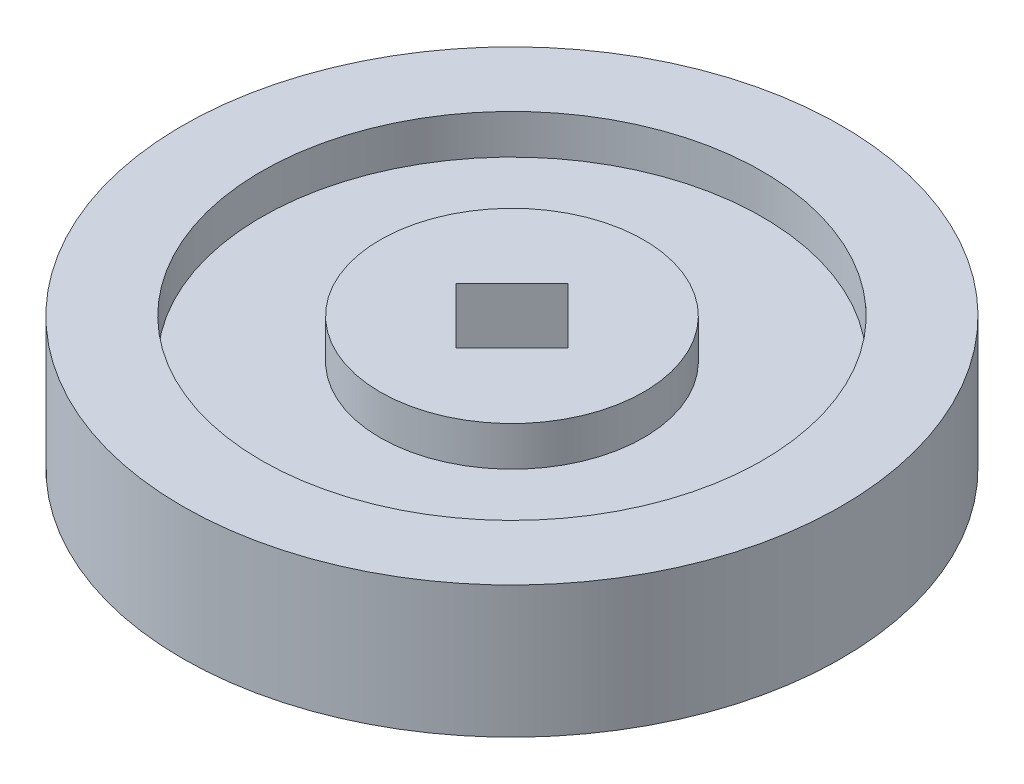
from build123d import *

# Parameters (mm, degrees)
SKETCH1_R           = 25
SKETCH1_R_2         = 19
BOSS_EXTRUDE1_DEPTH = 5
SKETCH2_R           = 10
BOSS_EXTRUDE2_DEPTH = 12
SKETCH3_R           = 19
SKETCH3_R_2         = 10
BOSS_EXTRUDE3_DEPTH = 2
CUT_EXTRUDE1_DEPTH  = 50


with BuildPart() as part:
    # Sketch1 → Boss-Extrude1 (new, symmetric)
    with BuildSketch(Plane(origin=(0, 0, 0), x_dir=(1, 0, 0), z_dir=(0, 1, 0))):
        with Locations(Location((0, 0, 0), (0, 0, 270))):
            Circle(SKETCH1_R)
        with Locations(Location((0, 0, 0), (0, 0, 270))):
            Circle(SKETCH1_R_2, mode=Mode.SUBTRACT)
    extrude(amount=BOSS_EXTRUDE1_DEPTH, both=True)



with BuildPart() as body_2:
    # Sketch2 → Boss-Extrude2 (new body)
    with BuildSketch(Plane(origin=(0, 5, 0), x_dir=(1, 0, 0), z_dir=(0, 1, 0))):
        with Locations(Location((0, 0, 0), (0, 0, 270))):
            Circle(SKETCH2_R)
    extrude(amount=-BOSS_EXTRUDE2_DEPTH)


with BuildPart() as part_1:
    add(part.part)

    add(body_2.part)  # Boss-Extrude3 merges body 2
    # Sketch3 → Boss-Extrude3 (add, symmetric)
    with BuildSketch(Plane(origin=(0, 0, 0), x_dir=(1, 0, 0), z_dir=(0, 1, 0))):
        with Locations(Location((0, 0, 0), (0, 0, 270))):
            Circle(SKETCH3_R)
        with Locations(Location((0, 0, 0), (0, 0, 270))):
            Circle(SKETCH3_R_2, mode=Mode.SUBTRACT)
    extrude(amount=BOSS_EXTRUDE3_DEPTH, both=True)

    # Sketch4 → Cut-Extrude1 (cut)
    with BuildSketch(Plane.XZ.offset(7)):
        Polygon((-4.242640687, 0), (0, 4.242640687), (4.242640687, 0), (0, -4.242640687), align=None)
    extrude(amount=-CUT_EXTRUDE1_DEPTH, mode=Mode.SUBTRACT)


solid = part_1.part
